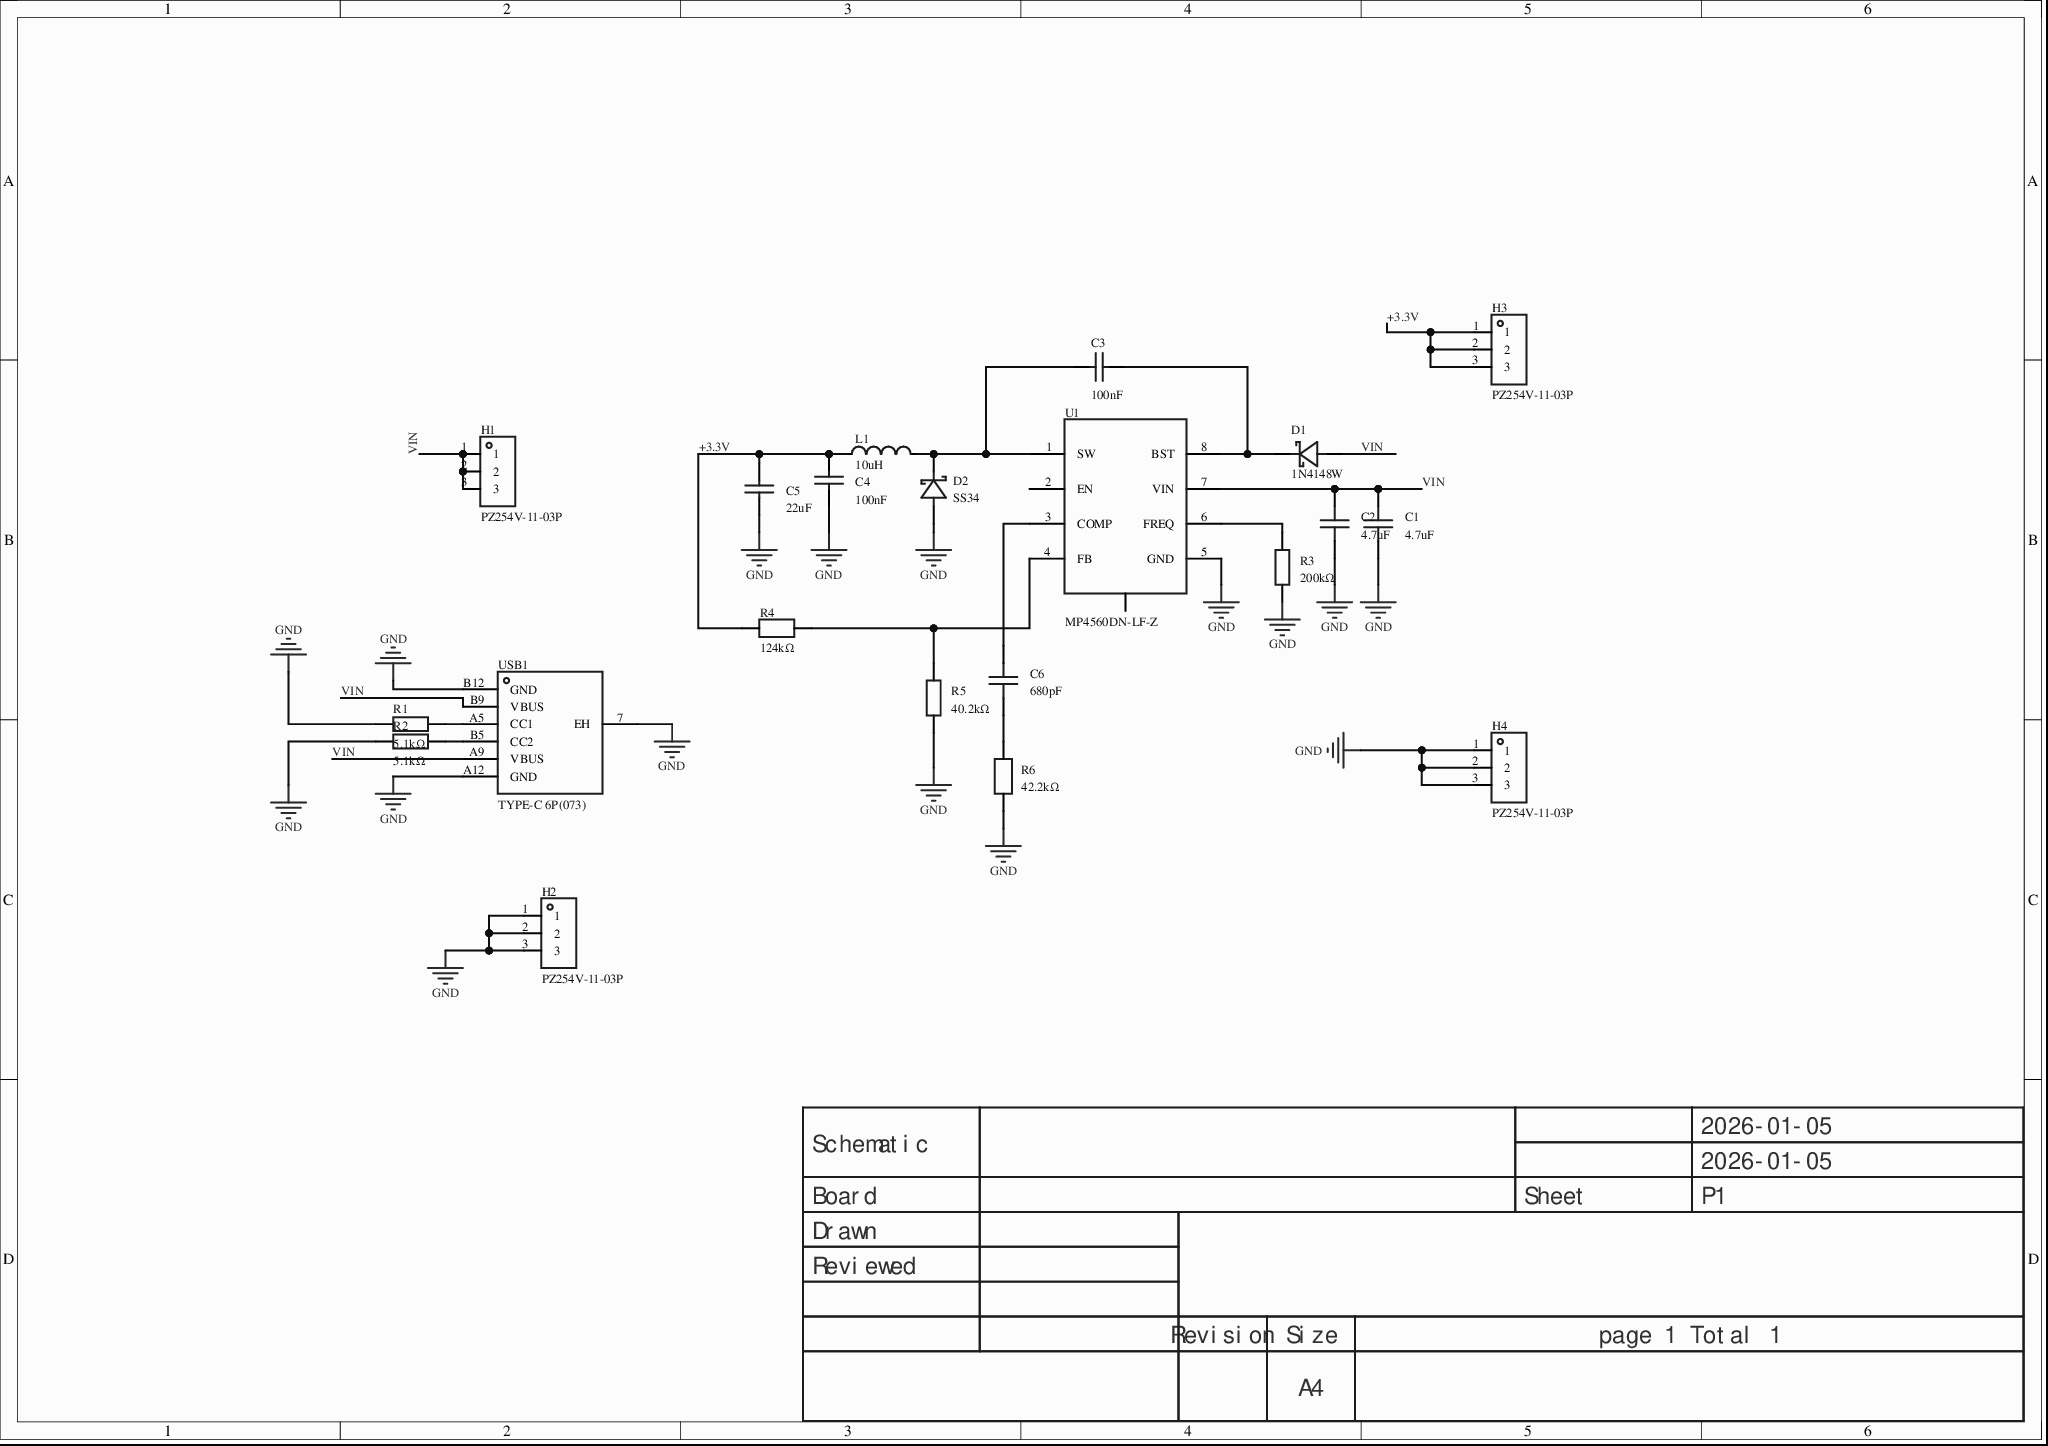
[diagram p0: MISC51170-3.schdoc]
# Altium project MISC51170-2.PrjPcb
1 sheet, 21 parts. Net scope: global (net labels, ports and power ports of the same name join across sheets).
Board file: MISC51170.pcbdoc

## Sheet MISC51170-3.schdoc
size 297 x 209 mm; Version: V1.0; @Project Name: MISC51170; @Update Date: 2026-01-05; @Create Date: 2026-01-05; @Board Name: MISC51170; @Create Time: 10:05:42; @Page Count: 1; @Page No: 1; @Schematic Name: MISC51170; @Update Time: 10:05:42; Size: A4

### Parts
C1  4.7uF  [C1206]
C2  4.7uF  [C1206]
C3  100nF  [C0805]
C4  100nF  [C0805]
C5  22uF  [C1206]
C6  680pF  [C0805]
D1  1N4148W  [SOD-123_L2.7-W1.6-LS3.7-FD]
D2  SS34  [SMA_L4.3-W2.6-LS5.0-FD]
H1  PZ254V-11-03P  [HDR-TH_3P-P2.54-V-M_PZ254V-11-03P]
H2  PZ254V-11-03P  [HDR-TH_3P-P2.54-V-M_PZ254V-11-03P]
H3  PZ254V-11-03P  [HDR-TH_3P-P2.54-V-M_PZ254V-11-03P]
H4  PZ254V-11-03P  [HDR-TH_3P-P2.54-V-M_PZ254V-11-03P]
L1  10uH  [IND-SMD_L5.2-W5.2_MCW-0530]
R1  5.1kΩ  [R0805]
R2  5.1kΩ  [R0805]
R3  200kΩ  [R0805]
R4  124kΩ  [R0805]
R5  40.2kΩ  [R0805]
R6  42.2kΩ  [R0805]
U1  MP4560DN-LF-Z  [SOIC-8_L4.9-W3.9-P1.27-LS6.0-BL-EP3.1-1]
USB1  TYPE-C 6P(073)  [TYPE-C-SMD_TYPE-C-6P-073]

### Nets
GND: C1.2 C2.2 C4.2 C5.1 D2.1(A) H2.1 H2.2 H2.3 H4.1 H4.2 H4.3 R1.1 R2.1 R3.2 R5.2 R6.1 U1.5(GND) USB1.7(EH) USB1.A12(GND) USB1.B12(GND)
+3.3V: C4.1 C5.2 H3.1 H3.2 H3.3 L1.1 R4.1
VIN: C1.1 C2.1 D1.1(A) H1.1 H1.2 H1.3 U1.7(VIN) USB1.A9(VBUS) USB1.B9(VBUS)
NetC3_1: C3.1 D1.2(K) U1.8(BST)
NetC3_2: C3.2 D2.2(K) L1.2 U1.1(SW)
NetC6_1: C6.1 R6.2
NetC6_2: C6.2 U1.3(COMP)
NetR1_2: R1.2 USB1.A5(CC1)
NetR2_2: R2.2 USB1.B5(CC2)
NetR3_1: R3.1 U1.6(FREQ)
NetR4_2: R4.2 R5.1 U1.4(FB)

Not connected (* = marked no-connect by the designer): U1 2(EN)* 9

### Notes on the sheet
- 2026-01-05
- Schematic
- Board
- Sheet
- P1
- Drawn
- Reviewed
- Revision
- Size
- A4
- page 1 Total 1

### Library data of the parts
C1 C2 = GRM31CC72A475KE11L: Capacitance: 4.7uF; tolerance: ±10%; rated voltage: 100V; temperature coefficient: X7S;; Manufacturer: muRata(村田); AddInBom: yes; ModelId: e4be705b945545a48e666415e3682bd80819f05c4eef4c71ace90d822a990e87; ModelName: C1206_L3.2-W1.6-H1.3; ModelTransform: 125.984,62.992,0,0,0,0,0,0,0; Symbol: GRM31CC72A475KE11L; Device: GRM31CC72A475KE11L; LCSC Part Name: 4.7uF ±10% 100V; SupplierPart: C237304; ManufacturerPart: GRM31CC72A475KE11L; Supplier Footprint: 1206; JLCPCB Part Class: Extended Part; Datasheet: https://item.szlcsc.com/datasheet/GRM31CC72A475KE11L/236748.html; Supplier: LCSC; ConvertToPcb: yes; FootprintName: C1206; Value: 4.7uF; Tolerance: ±10%; Voltage Rating: 100V; Temperature Coefficient: X7S
C3 C4 = CL21B104KCFNNNE: Capacitance: 100nF; tolerance: ±10%; rated voltage: 100V; temperature coefficient: X7R;; Manufacturer: SAMSUNG(三星); AddInBom: yes; ModelId: 1ba041120af144c991958decab20d2410819f05c4eef4c71ace90d822a990e87; ModelName: C0805_L2.0-W1.3-H1.3; ModelTransform: 78.74,51.181,0,0,0,0,0,0.0005,0; Symbol: CL21B104KCFNNNE; Device: CL21B104KCFNNNE; LCSC Part Name: 100nF ±10% 100V; SupplierPart: C28233; ManufacturerPart: CL21B104KCFNNNE; Supplier Footprint: 0805; JLCPCB Part Class: Basic Part; Datasheet: https://item.szlcsc.com/datasheet/CL21B104KCFNNNE/28983.html; Supplier: LCSC; ConvertToPcb: yes; FootprintName: C0805; Value: 100nF; Tolerance: ±10%; Voltage Rating: 100V; Temperature Coefficient: X7R
C5 = CL31A226KAHNNNE: Capacitance: 22uF; tolerance: ±10%; rated voltage: 25V; temperature coefficient: X5R;; Manufacturer: SAMSUNG(三星); AddInBom: yes; ModelId: e4be705b945545a48e666415e3682bd80819f05c4eef4c71ace90d822a990e87; ModelName: C1206_L3.2-W1.6-H1.3; ModelTransform: 125.984,62.992,0,0,0,0,0,0,0; Symbol: CL31A226KAHNNNE; Device: CL31A226KAHNNNE; LCSC Part Name: 22uF ±10% 25V; SupplierPart: C12891; ManufacturerPart: CL31A226KAHNNNE; Supplier Footprint: 1206; JLCPCB Part Class: Basic Part; Datasheet: https://item.szlcsc.com/datasheet/CL31A226KAHNNNE/13537.html; Supplier: LCSC; ConvertToPcb: yes; FootprintName: C1206; Value: 22uF; Tolerance: ±10%; Voltage Rating: 25V; Temperature Coefficient: X5R
C6 = CGA0805C0G681J500HT: Capacitance: 680pF; tolerance: ±5%; rated voltage: 50V; temperature coefficient: C0G;; Manufacturer: HRE(芯声); AddInBom: yes; ModelId: 1ba041120af144c991958decab20d2410819f05c4eef4c71ace90d822a990e87; ModelName: C0805_L2.0-W1.3-H1.3; ModelTransform: 78.74,51.181,0,0,0,0,0,0.0005,0; Symbol: CGA0805C0G681J500HT; Device: CGA0805C0G681J500HT; LCSC Part Name: 680pF ±5% 50V; SupplierPart: C22470029; ManufacturerPart: CGA0805C0G681J500HT; Supplier Footprint: 0805; JLCPCB Part Class: Extended Part; Datasheet: https://item.szlcsc.com/datasheet/CGA0805C0G681J500HT/24184525.html; Supplier: LCSC; ConvertToPcb: yes; FootprintName: C0805; Value: 680pF; Tolerance: ±5%; Voltage Rating: 50V; Temperature Coefficient: C0G
D1 = 1N4148W_C7420318: Diode configuration: discrete; forward voltage (Vf): 1.25V@150mA; DC reverse voltage (Vr): 100V; rectified current: 150mA; reverse recovery time (Trr): 4ns;; Manufacturer: R+O(宏嘉诚); AddInBom: yes; ModelId: 5054d9b7be8b429dad093a54b517b4dd0819f05c4eef4c71ace90d822a990e87; ModelTransform: 145.669,61.024,0,0,0,0,0,0,0; Pd - Power Dissipation: 400mW; Reverse Leakage Current (Ir): 1uA@75V; Operating Junction Temperature Range: -55℃~+150℃; Non-Repetitive Peak Forward Surge Current: 2A; Symbol: 1N4148W_C7420318; Device: 1N4148W_C7420318; LCSC Part Name: 100V 150mA; SupplierPart: C7420318; ManufacturerPart: 1N4148W; Supplier Footprint: SOD-123; JLCPCB Part Class: Extended Part; Datasheet: https://item.szlcsc.com/datasheet/1N4148W/8397140.html; Supplier: LCSC; ConvertToPcb: yes; FootprintName: SOD-123_L2.7-W1.6-LS3.7-FD; ModelName: SOD-123_L2.7-W1.6-LS3.7-FD; Diode Configuration: Discrete; Voltage - Forward(Vf@If): 1.25V@150mA; Voltage - DC Reverse(Vr): 100V; Current - Rectified: 150mA; Reverse Recovery Time (trr): 4ns
D2 = SS34_C7420365: Diode configuration: discrete; forward voltage (Vf): 550mV@3.0A; DC reverse voltage (Vr): 40V; rectified current: 3A;; Manufacturer: R+O(宏嘉诚); AddInBom: yes; ModelId: 7e24bebe6cd74171ae8c9de6fc5b78aa0819f05c4eef4c71ace90d822a990e87; ModelTransform: 198.4248,103.5431,0,180,0,0,-0.001,0,0; Reverse Leakage Current (Ir): 200uA@40V; Symbol: SS34_C7420365; Device: SS34_C7420365; LCSC Part Name: 电压:40V 电流:3A; SupplierPart: C7420365; ManufacturerPart: SS34; Supplier Footprint: SMA(DO-214AC); JLCPCB Part Class: Extended Part; Datasheet: https://item.szlcsc.com/datasheet/SS34/8397187.html; Supplier: LCSC; ConvertToPcb: yes; FootprintName: SMA_L4.3-W2.6-LS5.0-FD; ModelName: SMA_L4.3-W2.6-LS5.0-FD; Diode Configuration: Discrete; Voltage - Forward(Vf@If): 550mV@3.0A; Voltage - DC Reverse(Vr): 40V; Current - Rectified: 3A
H1-H4 = PZ254V-11-03P: Pin structure: 1x3P; pitch: 2.54mm; row spacing: -; round/square pin: square pin; mounting: through-hole; rows: single row; total pins: 3P; rated current: 3A; rated voltage: 250V; mating pin length: 6mm; plastic height: 2.5mm; termination pin length: 3mm; operating temperature: -40℃~+105℃; colour: black;; Manufacturer: XFCN(兴飞); Symbol: PZ254V-11-03P_C2937625; AddInBom: yes; Device: PZ254V-11-03P; LCSC Part Name: 1x3P 间距:2.54mm 方针 直插; SupplierPart: C2937625; ManufacturerPart: PZ254V-11-03P; Supplier Footprint: 插件,P=2.54mm; JLCPCB Part Class: Extended Part; Datasheet: https://item.szlcsc.com/datasheet/PZ254V-11-03P/3293280.html; Supplier: LCSC; ConvertToPcb: yes; FootprintName: HDR-TH_3P-P2.54-V-M_PZ254V-11-03P; Pin Structure: 1x3P; Pitch: 2.54mm; Row Spacing: -; Circluar Pins/Square Pins: Square; Mounting Type: Through-hole; Number of Rows: Single row; Number of Pins: 3P; Current Rating: 3A; Voltage Rating (Max): 250V; Length of Mating Pin: 6mm; Insulation Height: 2.5mm; Length of End Connection Pin: 3mm; Operating Temperature: -40℃~+105℃; Color: Black
L1 = SMMS0530-100M: Inductance: 10uH; tolerance: ±20%; rated current: 3.2A; saturation current (Isat): 3.5A; type: -;; Manufacturer: SXN(顺翔诺); AddInBom: yes; ModelId: b4c522bd73b14c1ca1c7df39bce432c30819f05c4eef4c71ace90d822a990e87; ModelName: IND-SMD_L5.4-W5.2-H3.0_MCW-0530; ModelTransform: 212.598,204.724,0,0,0,0,0,0,0; DC Resistance(DCR): 125mΩ; Symbol: SMMS0530-100M; Device: SMMS0530-100M; LCSC Part Name: 10uH ±20% 3.5A; SupplierPart: C181721; ManufacturerPart: SMMS0530-100M; Supplier Footprint: SMD,5.5x5.2mm; JLCPCB Part Class: Extended Part; Datasheet: https://item.szlcsc.com/datasheet/SMMS0530-100M/193118.html; Supplier: LCSC; ConvertToPcb: yes; FootprintName: IND-SMD_L5.2-W5.2_MCW-0530; Value: 10uH; Tolerance: ±20%; Current Rating: 3.2A; Current - Saturation(Isat): 3.5A; Type: -
R1 R2 = 0805W8F5101T5E: Resistor type: thick film resistor; resistance: 5.1kΩ; tolerance: ±1%; power: 125mW; working voltage: 150V; temperature coefficient: ±100ppm/℃;; Manufacturer: UNI-ROYAL(厚声); AddInBom: yes; ModelId: 37a81e68749a4138bd2dfa6897b24b850819f05c4eef4c71ace90d822a990e87; ModelName: R0805_L2.0-W1.3-H0.6; ModelTransform: 78.74,51.181,0,0,0,0,0,-0.0005,0; Symbol: 0805W8F5101T5E; Device: 0805W8F5101T5E; LCSC Part Name: 5.1kΩ ±1% 125mW 厚膜电阻; SupplierPart: C27834; ManufacturerPart: 0805W8F5101T5E; Supplier Footprint: 0805; JLCPCB Part Class: Basic Part; Datasheet: https://item.szlcsc.com/datasheet/0805W8F5101T5E/28584.html; Supplier: LCSC; ConvertToPcb: yes; FootprintName: R0805; Type: Thick film resistor; Value: 5.1kΩ; Tolerance: ±1%; Power(Watts): 125mW; Voltage-Supply(Max): 150V; Temperature Coefficient: ±100ppm/℃; Operating Temperature: -55℃~+155℃
R3 = 0805W8F2003T5E: Resistor type: thick film resistor; resistance: 200kΩ; tolerance: ±1%; power: 125mW; max working voltage: 150V; temperature coefficient: ±100ppm/℃;; Manufacturer: UNI-ROYAL(厚声); AddInBom: yes; ModelId: 37a81e68749a4138bd2dfa6897b24b850819f05c4eef4c71ace90d822a990e87; ModelName: R0805_L2.0-W1.3-H0.6; ModelTransform: 78.74,51.181,0,0,0,0,0,-0.0005,0; Symbol: 0805W8F2003T5E; Device: 0805W8F2003T5E; LCSC Part Name: 200kΩ ±1% 125mW 厚膜电阻; SupplierPart: C17539; ManufacturerPart: 0805W8F2003T5E; Supplier Footprint: 0805; JLCPCB Part Class: Basic Part; Datasheet: https://atta.szlcsc.com/upload/public/pdf/source/20200306/C422600_1E6D84923E4A46A82E41ADD87F860B5C.pdf; Supplier: LCSC; ConvertToPcb: yes; FootprintName: R0805; Type: Thick film resistor; Value: 200kΩ; Tolerance: ±1%; Power(Watts): 125mW; Overload Voltage (Max): 150V; Temperature Coefficient: ±100ppm/℃; Operating Temperature Range: -55℃~+155℃
R4 = FRC0805F1243TS: Resistor type: thick film resistor; resistance: 124kΩ; tolerance: ±1%; power: 125mW; working voltage: 150V; temperature coefficient: ±100ppm/℃;; Manufacturer: FOJAN(富捷); AddInBom: yes; ModelId: 37a81e68749a4138bd2dfa6897b24b850819f05c4eef4c71ace90d822a990e87; ModelName: R0805_L2.0-W1.3-H0.6; ModelTransform: 78.74,51.181,0,0,0,0,0,-0.0005,0; Symbol: FRC0805F1243TS; Device: FRC0805F1243TS; LCSC Part Name: 124kΩ ±1% 125mW 厚膜电阻; SupplierPart: C2933298; ManufacturerPart: FRC0805F1243TS; Supplier Footprint: 0805; JLCPCB Part Class: Extended Part; Supplier: LCSC; ConvertToPcb: yes; FootprintName: R0805; Type: Thick film resistor; Value: 124kΩ; Tolerance: ±1%; Power(Watts): 125mW; Voltage-Supply(Max): 150V; Temperature Coefficient: ±100ppm/℃; Operating Temperature: -55℃~+155℃
R5 = 0805W8F4022T5E: Resistor type: thick film resistor; resistance: 40.2kΩ; tolerance: ±1%; power: 125mW; working voltage: 150V; temperature coefficient: ±100ppm/℃;; Manufacturer: UNI-ROYAL(厚声); AddInBom: yes; ModelId: 37a81e68749a4138bd2dfa6897b24b850819f05c4eef4c71ace90d822a990e87; ModelName: R0805_L2.0-W1.3-H0.6; ModelTransform: 78.74,51.181,0,0,0,0,0,-0.0005,0; Symbol: 0805W8F4022T5E; Device: 0805W8F4022T5E; LCSC Part Name: 40.2kΩ ±1% 125mW 厚膜电阻; SupplierPart: C17678; ManufacturerPart: 0805W8F4022T5E; Supplier Footprint: 0805; JLCPCB Part Class: Extended Part; Datasheet: https://item.szlcsc.com/datasheet/0805W8F4022T5E/18366.html; Supplier: LCSC; ConvertToPcb: yes; FootprintName: R0805; Type: Thick film resistor; Value: 40.2kΩ; Tolerance: ±1%; Power(Watts): 125mW; Voltage-Supply(Max): 150V; Temperature Coefficient: ±100ppm/℃; Operating Temperature: -55℃~+155℃
R6 = FRC0805F4222TS: Resistor type: thick film resistor; resistance: 42.2kΩ; tolerance: ±1%; power: 125mW; working voltage: 150V; temperature coefficient: ±100ppm/℃;; Manufacturer: FOJAN(富捷); AddInBom: yes; ModelId: 37a81e68749a4138bd2dfa6897b24b850819f05c4eef4c71ace90d822a990e87; ModelName: R0805_L2.0-W1.3-H0.6; ModelTransform: 78.74,51.181,0,0,0,0,0,-0.0005,0; Symbol: FRC0805F4222TS; Device: FRC0805F4222TS; LCSC Part Name: 42.2kΩ ±1% 125mW 厚膜电阻; SupplierPart: C2999591; ManufacturerPart: FRC0805F4222TS; Supplier Footprint: 0805; JLCPCB Part Class: Extended Part; Datasheet: https://item.szlcsc.com/datasheet/FRC0805F4222TS/3477031.html; Supplier: LCSC; ConvertToPcb: yes; FootprintName: R0805; Type: Thick film resistor; Value: 42.2kΩ; Tolerance: ±1%; Power(Watts): 125mW; Voltage-Supply(Max): 150V; Temperature Coefficient: ±100ppm/℃; Operating Temperature: -55℃~+155℃
U1 = MP4560DN-LF-Z: Function type: buck; output type: adjustable; working voltage: 3.8V~55V; output voltage: 800mV~52V; output current: 2A;; Manufacturer: MPS(芯源); Symbol: MP4560DN–LF–Z; AddInBom: yes; ModelId: 2424bcfd05224efdb78db06799097c7b0819f05c4eef4c71ace90d822a990e87; ModelTransform: 192.913,236.22,0,0,0,0,0,0,0; Frequency - Switching: 1MHz; 2MHz; Synchronous Rectifier: No; Number of Outputs: 1; Quiescent Current: 140uA; Switch tube (built-in/external): Built-in; Device: MP4560DN-LF-Z; LCSC Part Name: 2A, 2MHz, 55V降压转换器; SupplierPart: C40133; ManufacturerPart: MP4560DN-LF-Z; Supplier Footprint: SOIC-8-EP; JLCPCB Part Class: Extended Part; Datasheet: https://item.szlcsc.com/datasheet/MP4560DN-LF-Z/41115.html; Supplier: LCSC; ConvertToPcb: yes; FootprintName: SOIC-8_L4.9-W3.9-P1.27-LS6.0-BL-EP3.1-1; ModelName: SOIC-8_L4.9-W3.9-P1.27-LS6.0-BL-EP3.1-1; Function: Buck; Output Type: Adjustable; Voltage - Supply: 3.8V~55V; Output Voltage: 800mV~52V; Output Current: 2A; Operating Temperature: -40℃~+125℃@(TJ); Topology: Buck
USB1 = TYPE-C 6P(073): Connector type: Type-C; standard: USB 3.1; gender: female; mounting: horizontal SMT; contacts: 6P; ports: 1; rated current - power: 3A; operating temperature: -25℃~+85℃;; Manufacturer: SHOU HAN(首韩); AddInBom: yes; ModelId: 5572357f2a5242b0b12e4512f7b213ab0819f05c4eef4c71ace90d822a990e87; ModelTransform: 351.968,281.49546,0,0,0,0,0.002,-46.967,-39.37; Number of Ports: 1; Rated Voltage (Max): 5V; Connect-Disconnect Life: 1万次; Core Colour: Black; Symbol: TYPE-C 6P(073); Device: TYPE-C 6P(073); LCSC Part Name: Type-C 母 卧贴; SupplierPart: C668623; ManufacturerPart: TYPE-C 6P(073); Supplier Footprint: SMD; JLCPCB Part Class: Extended Part; Datasheet: https://atta.szlcsc.com/upload/public/pdf/source/20200618/C668623_A4B260DED7AC1949BAC6AE39E9F4CD80.pdf; Supplier: LCSC; ConvertToPcb: yes; FootprintName: TYPE-C-SMD_TYPE-C-6P-073; ModelName: TYPE-C-SMD_TYPE-C-6P-073; Connector Type: Type-C; Standard: USB 3.1; Gender: Female; Mounting Style: Horizontal SMT; Number of Contacts: 6P; Current Rating - Power (Max): 3A; Operating Temperature Range: -25℃~+85℃